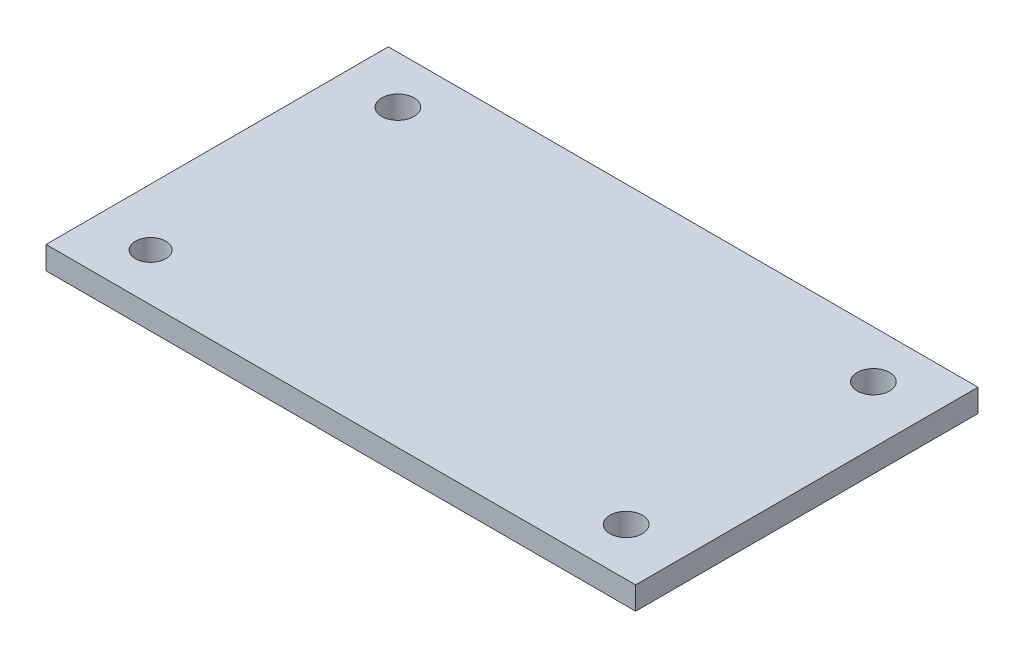
from build123d import *

# Parameters (mm, degrees)
SKETCH1_W      = 310
SKETCH1_H      = 180
SKETCH1_R      = 8.5
SKETCH1_R_2    = 8
EXTRUDE1_DEPTH = 6


with BuildPart() as part:
    # Sketch1 → Extrude1 (new, symmetric)
    with BuildSketch(Plane(origin=(0, 0, 0), x_dir=(1, 0, 0), z_dir=(0, 1, 0))):
        Rectangle(SKETCH1_W, SKETCH1_H)
        with Locations(Location((125, -65, 0), (0, 0, 270))):
            Circle(SKETCH1_R, mode=Mode.SUBTRACT)
        with Locations(Location((-125, -65, 0), (0, 0, 270))):
            Circle(SKETCH1_R_2, mode=Mode.SUBTRACT)
        with Locations(Location((-125, 65, 0), (0, 0, 270))):
            Circle(SKETCH1_R, mode=Mode.SUBTRACT)
        with Locations(Location((125, 65, 0), (0, 0, 270))):
            Circle(SKETCH1_R, mode=Mode.SUBTRACT)
    extrude(amount=EXTRUDE1_DEPTH, both=True)


solid = part.part
